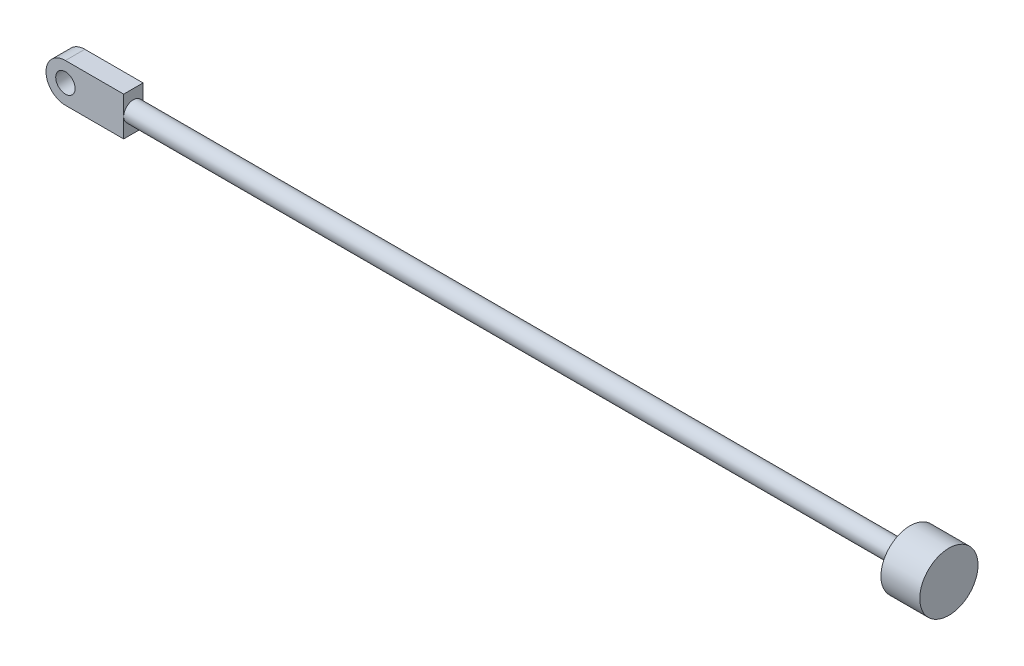
SolidWorks part; units mm, degrees
material "普通碳钢"
ref_plane "Front Plane" through (0, 0, 0) normal (0, 0, 1) x (1, 0, 0)
ref_plane "Top Plane" through (0, 0, 0) normal (0, 1, 0) x (1, 0, 0)
ref_plane "Right Plane" through (0, 0, 0) normal (1, 0, 0) x (0, 0, -1)
sketch "Sketch1" plane through (0, 0, 0) normal (0, 0, 1) x (1, 0, 0)
  line L0 (0, 10) -> (30, 10)
  line L1 (30, 10) -> (30, -10)
  line L2 (30, -10) -> (0, -10)
  circle A0 centre (0, 0) radius 5
  arc A1 (0, 10) -> (0, -10) centre (0, 0) ccw
  dimension "D1" = 10
  dimension "D2" = 20
  dimension "D3" = 30
extrude "Boss-Extrude1" add sketch "Sketch1" along normal mid plane 10
sketch "Sketch2" plane through (0, 0, 0) normal (0, 0, 1) x (1, 0, 0)
  line L0 (30, 0) -> (30, -5)
  line L2 (30, -5) -> (430, -5)
  line L3 (30, -10) -> (30, 10) construction
  line L4 (430, -5) -> (430, -15)
  line L5 (430, -15) -> (450, -15)
  line L6 (450, -15) -> (450, 0)
  line L7 (450, 0) -> (30, 0)
  dimension "D1" = 5
  dimension "D2" = 420
  dimension "D3" = 15
  dimension "D4" = 20
revolve "Revolve1" add sketch "Sketch2" angle 360 about L7
